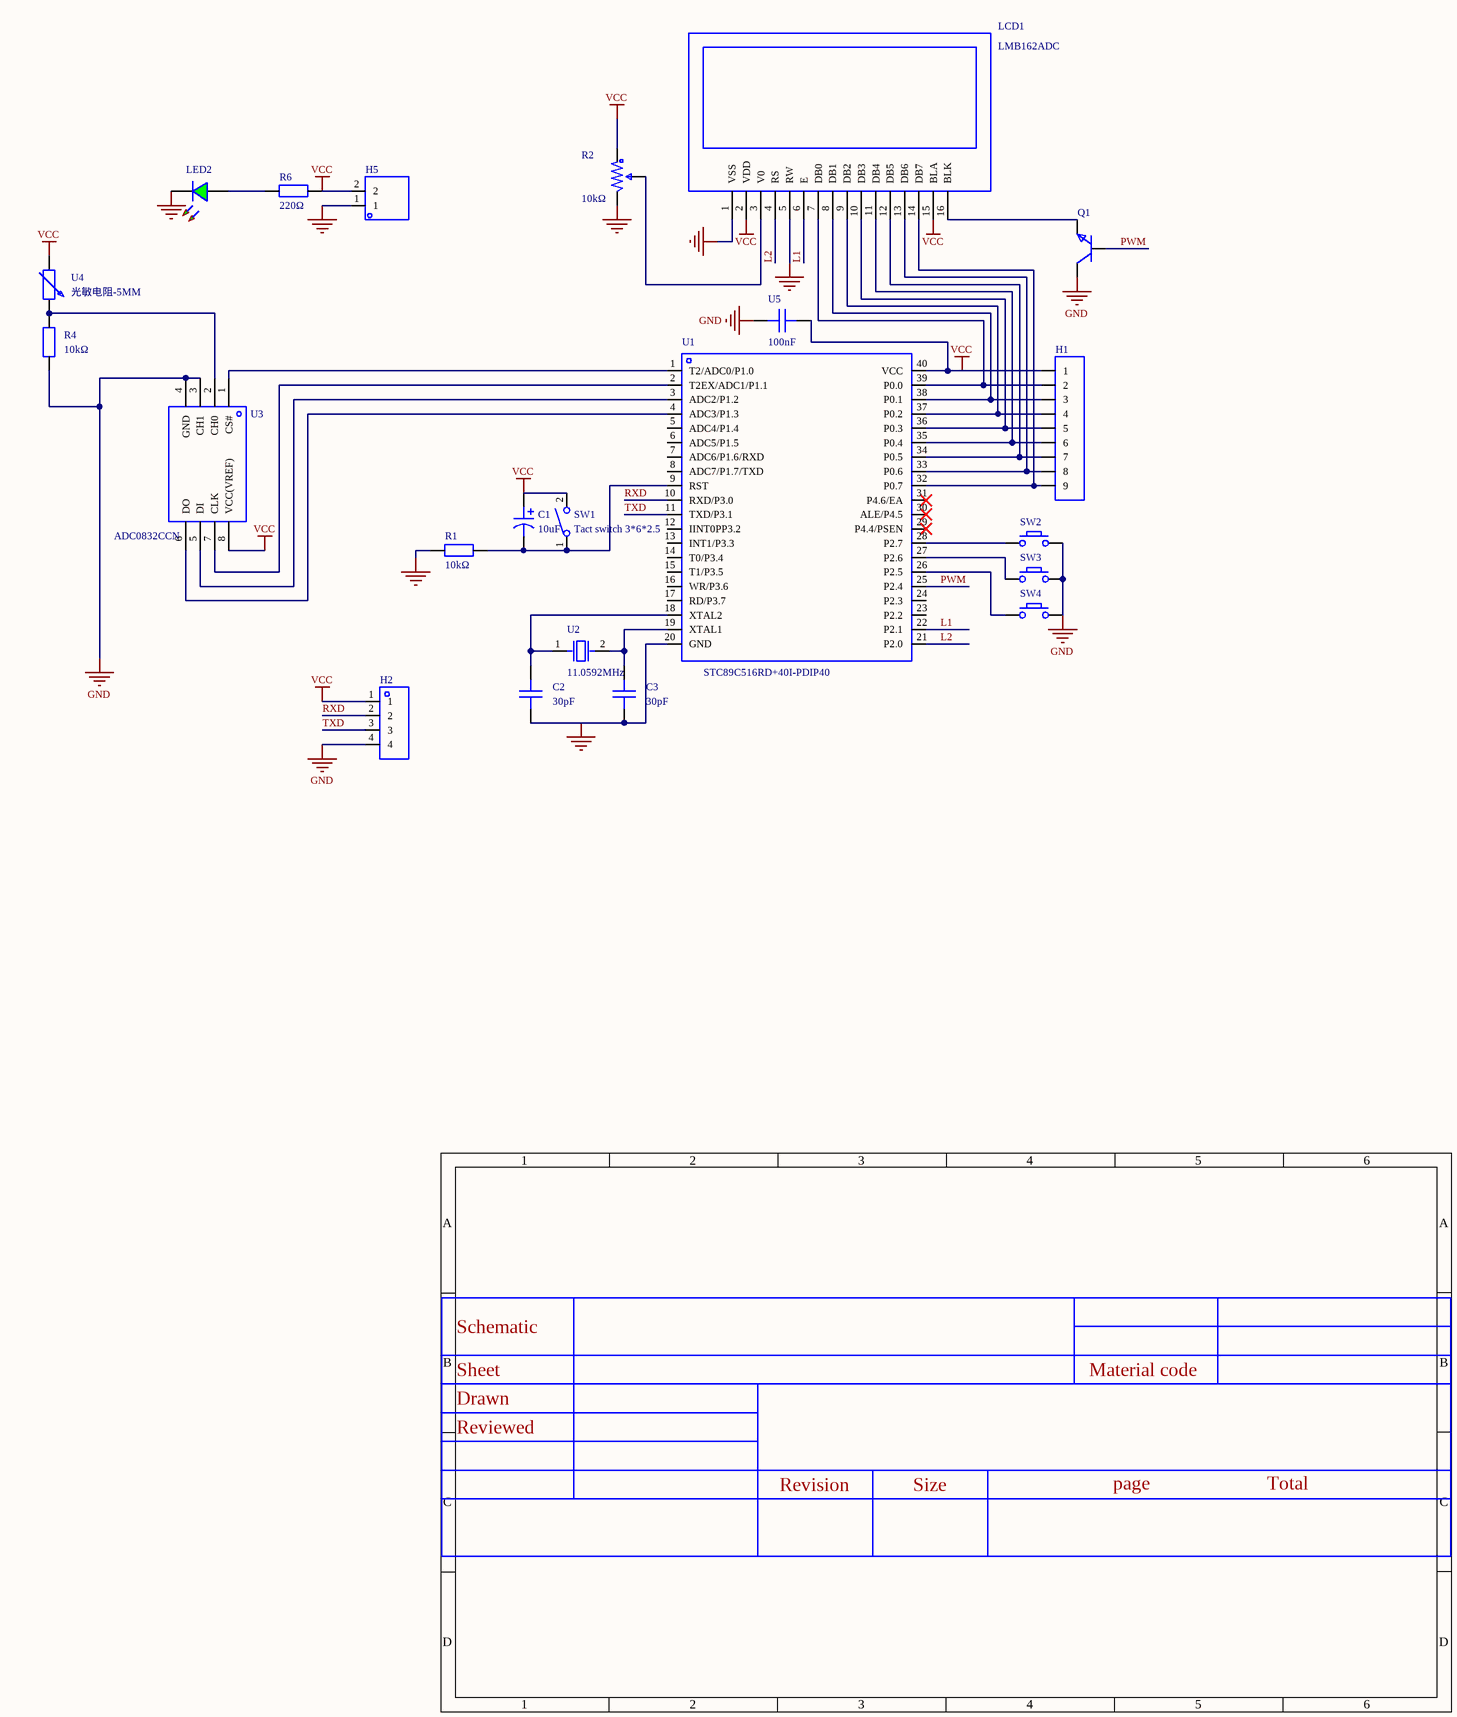
[diagram p0: MISC51926-3.schdoc]
# Altium project MISC51926-2.PrjPcb
1 sheet, 22 parts. Net scope: global (net labels, ports and power ports of the same name join across sheets).
Board file: MISC51926.pcbdoc

## Sheet MISC51926-3.schdoc
size 178 x 98 mm; Version: V1.0; @Project Name: MISC51926; @Page Count: 1; @Update Date: 2026-04-15; @Create Date: 2026-04-15; @Schematic Name: MISC51926; @Page No: 1; @Board Name: MISC51926; @Create Time: 22:37:32; @Update Time: 22:37:32

### Parts
C1  10uF  [CAP-TH_BD5.0-P2.00-D0.8-FD-10UF50VC110GL]
C2  30pF  [CAP-TH_L3.8-W2.5-P2.54-D0.50]
C3  30pF  [CAP-TH_L3.8-W2.5-P2.54-D0.50]
H1  (no value)  [HDR-TH_9P-P2.54-V-F-1]
H2  (no value)  [HDR-TH_4P-P2.54-V-M]
H5  (no value)  [HDR-TH_2P-P2.54-V-M-1]
LCD1  LMB162ADC  [LCD1602]
LED2  (no value)  [LED_TH-3mm]
Q1  (no value)  [S8050_SOT-23]
R1  10kΩ  [Res_1/8W]
R2  10kΩ  [RES-ADJ-SMD_RM065-V1]
R4  10kΩ  [Res_1/8W]
R6  220Ω  [Res_1/8W]
SW1  Tact switch 3*6*2.5  [SW-SMD_L6.0-W3.6-LS8.0]
SW2  (no value)  [Key_TH_3.5x6x4.3]
SW3  (no value)  [Key_TH_3.5x6x4.3]
SW4  (no value)  [Key_TH_3.5x6x4.3]
U1  STC89C516RD+40I-PDIP40  [DIP-40_L52.3-W13.9-P2.54-LS15.2-BL]
U2  11.0592MHz  [HC-49US_L11.0-W4.6-P4.88]
U3  ADC0832CCN  [DIP-8_L9.7-W6.4-P2.54-LS7.6-BL]
U4  光敏电阻-5MM  [RES-TH_L4.9-W4.3-P3.4]
U5  100nF  [CAP-TH_L5.0-W2.5-P5.00-D1.0]

### Nets
GND: C2.1 C3.1 H2.4 H5.1 LCD1.1(VSS) LCD1.5(RW) LED2.2(A) Q1.3 R1.1 R2.3 R4.1 SW2.B SW3.B SW4.B U1.20(GND) U3.3(CH1) U3.4(GND) U5.2
VCC: C1.1 H1.1 H2.1 H5.2 LCD1.2(VDD) LCD1.15(BLA) R2.1 R6.2 SW1.2 U1.40(VCC) U3.8(VCC(VREF)) U4.1 U5.1
L1: LCD1.6(E) U1.22(P2.1)
L2: LCD1.4(RS) U1.21(P2.0)
PWM: Q1.1 U1.25(P2.4)
RXD: H2.2 U1.10(RXD/P3.0)
TXD: H2.3 U1.11(TXD/P3.1)
NetC1_2: C1.2 R1.2 SW1.1 U1.9(RST)
NetC2_2: C2.2 U1.18(XTAL2) U2.1(OSC1)
NetC3_2: C3.2 U1.19(XTAL1) U2.2(OSC2)
NetH1_2: H1.2 LCD1.7(DB0) U1.39(P0.0)
NetH1_3: H1.3 LCD1.8(DB1) U1.38(P0.1)
NetH1_4: H1.4 LCD1.9(DB2) U1.37(P0.2)
NetH1_5: H1.5 LCD1.10(DB3) U1.36(P0.3)
NetH1_6: H1.6 LCD1.11(DB4) U1.35(P0.4)
NetH1_7: H1.7 LCD1.12(DB5) U1.34(P0.5)
NetH1_8: H1.8 LCD1.13(DB6) U1.33(P0.6)
NetH1_9: H1.9 LCD1.14(DB7) U1.32(P0.7)
NetLCD1_3: LCD1.3(V0) R2.2
NetLCD1_16: LCD1.16(BLK) Q1.2
NetLED2_1: LED2.1(C) R6.1
NetR4_2: R4.2 U3.2(CH0) U4.2
NetSW2_A: SW2.A U1.28(P2.7)
NetSW3_A: SW3.A U1.27(P2.6)
NetSW4_A: SW4.A U1.26(P2.5)
NetU1_1: U1.1(T2/ADC0/P1.0) U3.1(CS#)
NetU1_2: U1.2(T2EX/ADC1/P1.1) U3.7(CLK)
NetU1_3: U1.3(ADC2/P1.2) U3.5(DI)
NetU1_4: U1.4(ADC3/P1.3) U3.6(DO)

Not connected (* = marked no-connect by the designer): U1 5(ADC4/P1.4) 6(ADC5/P1.5) 7(ADC6/P1.6/RXD) 8(ADC7/P1.7/TXD) 12(IINT0PP3.2) 13(INT1/P3.3) 14(T0/P3.4) 15(T1/P3.5) 16(WR/P3.6) 17(RD/P3.7) 23(P2.2) 24(P2.3) 29(P4.4/PSEN)* 30(ALE/P4.5)* 31(P4.6/EA)*

### Notes on the sheet
- 2026-04-15
- Schematic
- Sheet
- Material code
- P1
- Reviewed
- Drawn
- 51 project
- Revision
- Size
- page
- Total
- A4
- 1

### Library data of the parts
C1 = 10UF50VC110GL: Capacitance: 10uF; tolerance: ±20%; rated voltage: 50V; ripple current: 120mA@100KHz; equivalent series resistance (ESR): 1.6Ω;; Manufacturer: Econd(米朗电子); AddInBom: yes; Pin Spacing: 2mm; Lifetime: 5000hrs@105℃; Symbol: 10UF50VC110GL; Device: 10UF50VC110GL; LCSC Part Name: 10uF ±20% 50V; SupplierPart: C46867109; ManufacturerPart: 10UF50VC110GL; Supplier Footprint: 插件,D5xL11mm; JLCPCB Part Class: Extended Part; Datasheet: https://item.szlcsc.com/datasheet/10UF50VC110GL/49031974.html; Supplier: LCSC; ConvertToPcb: yes; FootprintName: CAP-TH_BD5.0-P2.00-D0.8-FD-10UF50VC110GL; Value: 10uF; Tolerance: ±20%; Voltage Rating: 50V; Ripple Current: 120mA@100KHz; Equivalent Series Resistance(ESR): 1.6Ω; Diameter: 5mm; Height - Seated (Max): 11mm; Operating Temperature: -40℃~+105℃
C2 C3 = C315C300K3G5TA7301: Capacitance: 30pF; tolerance: ±10%; rated voltage: 25V; temperature coefficient: C0G;; Manufacturer: KEMET(基美); AddInBom: yes; ModelId: 0be8c650c9044d099e9add656cc6dda60819f05c4eef4c71ace90d822a990e87; ModelTransform: 149.606,98.8187,0,0,0,0,0,0,-196.85; Pin Spacing: 2.54mm; Symbol: C315C300K3G5TA7301; Device: C315C300K3G5TA7301; LCSC Part Name: 30pF ±10% 25V; SupplierPart: C2245291; ManufacturerPart: C315C300K3G5TA7301; Supplier Footprint: 插件,P=2.54mm; JLCPCB Part Class: Extended Part; Datasheet: https://item.szlcsc.com/datasheet/C315C300K3G5TA7301/2337370.html; Supplier: LCSC; ConvertToPcb: yes; FootprintName: CAP-TH_L3.8-W2.5-P2.54-D0.50; ModelName: CAP-TH_L3.8-W2.5-P2.54-D0.50; Value: 30pF; Tolerance: ±10%; Voltage Rating: 25V; Temperature Coefficient: C0G
H1 = HDR-F_2.54_1x9P: Symbol: Header-Female-2.54_1x9; AddInBom: yes; ModelId: 3a7016416d904017ac5ead6cc0f14e9c; ModelName: HDR-TH_9P-P2.54-F-LI-1X9P; ModelTransform: 915.746,94.488,0,0,0,0,0,0,-125.984; Device: HDR-F_2.54_1x9P; ConvertToPcb: yes; FootprintName: HDR-TH_9P-P2.54-V-F-1; SupplierPart: C39576; Supplier Footprint: 插件; JLCPCB Part Class: Extended Part
H2 = HDR-M_2.54_1x4P: Symbol: PZ254V-11-04P; 3D Model: 112f4d05e8d64e99ab9a333894bea4f9; 3D Model Transform: 399.999,104.7242,0,0,0,0,0,0,-118.11; ConvertToPcb: yes; ModelName: HDR-TH_4P-P2.54-M-LI-1X4P; Device: HDR-M_2.54_1x4P; Supplier Part: C492403; Supplier Footprint: 插件; AddInBom: yes; FootprintName: HDR-TH_4P-P2.54-V-M
H5 = HDR-M_2.54_1x2P: Symbol: 210S-1*2P L=11.6MMGold-plated black; ConvertToPcb: yes; ModelId: 79b2e9f2d70a4d68a1b7098f27c6d4c5; ModelName: HDR-M-2.54_1x2; ModelTransform: 200,100,0,0,0,0,0,0,-118.11; Device: HDR-M_2.54_1x2P; AddInBom: yes; SupplierPart: C124375; Supplier Footprint: 插件; FootprintName: HDR-TH_2P-P2.54-V-M-1
LCD1 = LMB162ADC: 16x2 character LCD module; AddInBom: yes; ModelId: f9d832f46a914cadb50fc4d4cefd2517; ModelTransform: 3149.6,1417.32,0,0,0,0,0,0,-118.11; Symbol: LMB162ADC; Device: LMB162ADC; LCSC Part Name: LMB162ADC; SupplierPart: C9741; ManufacturerPart: LMB162ADC; Supplier Footprint: SIP; JLCPCB Part Class: Extended Part; Supplier: LCSC; ConvertToPcb: yes; FootprintName: LCD1602; ModelName: LCD1602
LED2 = LED_TH-G_3mm: AddInBom: yes; ModelId: 07c881668c9448ef9b36eb6a2126ca130819f05c4eef4c71ace90d822a990e87; ModelName: LED-TH-3mm_G; ModelTransform: 141.27444,153.32669525336098,354.32999763315956,0,0,0,-5.90551,0,-137.79528; Symbol: LED_TH-G; Device: LED_TH-G_3mm; ConvertToPcb: yes; FootprintName: LED_TH-3mm; Supplier Footprint: 插件
Q1 = S8050_SOT_NPN: Symbol: NPN; ConvertToPcb: yes; ModelId: c62791f0466c4ae2a892c056b845b0ca0819f05c4eef4c71ace90d822a990e87; ModelName: SOT-23-3P_L2.9-W1.3-H1.0-LS2.4-P0.95; ModelTransform: 98.6,114.12,41.29,180,0,0,0,0,-3; Device: S8050_SOT_NPN; AddInBom: yes; Supplier Footprint: SOT-23; FootprintName: S8050_SOT-23
R1 R4 R6 = Res_AXIAL-1/8W: Symbol: Resistor; ConvertToPcb: yes; ModelId: b2b5ae7ae4c642178fe0039925c86a3f0819f05c4eef4c71ace90d822a990e87; ModelName: RES-TH_BD1.8-L3.2-P7.20-D0.4; ModelTransform: 282.86,66.88,253.09,0,0,0,0,0,-191; Device: Res_AXIAL-1/8W; AddInBom: yes; Supplier Footprint: 轴向引线; FootprintName: Res_1/8W
  R1 R4: Value: 10kΩ
  R6: Value: 220Ω
R2 = RM065-103(10K): Resistance: 10kΩ; tolerance: ±25%; power: 100mW;; Manufacturer: BOCHEN(博晨); AddInBom: yes; ModelId: c816c2b7942147f5a832150e8ef6960c0819f05c4eef4c71ace90d822a990e87; ModelTransform: 255.905,283.464,0,0,0,0,0.025,-3.937,-157.48; Voltage Rating: 50V; Symbol: RM065-103(10K); Device: RM065-103(10K); LCSC Part Name: 10kΩ ±25%; SupplierPart: C5205021; ManufacturerPart: RM065-103(10K); Supplier Footprint: 插件,7.3x6.4mm; JLCPCB Part Class: Extended Part; Datasheet: https://item.szlcsc.com/datasheet/RM065-103(10K)/5896379.html; Supplier: LCSC; ConvertToPcb: yes; FootprintName: RES-ADJ-SMD_RM065-V1; ModelName: RES-ADJ-SMD_RM065-V1; Value: 10kΩ; Tolerance: ±25%; Power(Watts): 100mW
SW1 = 轻触按键3*6*2.5: AddInBom: yes; ModelId: 5cda64a5897044e48badc24f5aa7d420; ModelName: SW-SMD_L6.0-W3.6-H2.5-LS8.0; ModelTransform: 314.96,141.732,0,0,0,0,0,0,0; Symbol: Tact switch 3*6*2.5; Device: Tact switch 3*6*2.5; LCSC Part Name: 轻触按键3*6*2.5; SupplierPart: C9900013040; ManufacturerPart: 轻触按键3*6*2.5; Supplier Footprint: KEY; JLCPCB Part Class: Extended Part; Supplier: LCSC; ConvertToPcb: yes; FootprintName: SW-SMD_L6.0-W3.6-LS8.0
SW2-SW4 = Key_TH_3.5x6x4.3: ConvertToPcb: yes; ModelId: c3523f9014d949d7ba5445190a3178990819f05c4eef4c71ace90d822a990e87; ModelName: SW-TH_L6.0-W3.5-H5.0-P6.5; ModelTransform: 308.49,137.8,335.08,0,0,0,0,0,-129.92; Symbol: Key_TH_3.5x6x4.3; Device: Key_TH_3.5x6x4.3; AddInBom: yes; Supplier Footprint: 插件; FootprintName: Key_TH_3.5x6x4.3
U1 = STC89C516RD+40I-PDIP40: CPU core: 51 series; program storage capacity: 61KB; RAM total capacity: 1.25KB; GPIO port count: 35; operating voltage range: 3.5V~5.5V; CPU max frequency: -; program memory type: FLASH;; Manufacturer: STC(宏晶); AddInBom: yes; ModelId: 16d4686a009b4ddca948f91eddb57b14; ModelName: DIP-40_L52.3-W13.8-H4.0-LS15.24-P2.54; ModelTransform: 2059.051,615.743,0,0,0,0,0,0,-129.921; GPIO Ports Number: 35; 16Bit Timer: 3; UART/USART: 1; Peripheral/Function: Watchdog; Symbol: STC89C516RD+40I-PDIP40; Device: STC89C516RD+40I-PDIP40; LCSC Part Name: STC89C516RD+40I-PDIP40; SupplierPart: C52225; ManufacturerPart: STC89C516RD+40I-PDIP40; Supplier Footprint: DIP-40; JLCPCB Part Class: Extended Part; Datasheet: https://atta.szlcsc.com/upload/public/pdf/source/20180614/C87831_BBAF7FB8B286C29ACE4E9B180C033FEC.pdf; Supplier: LCSC; ConvertToPcb: yes; FootprintName: DIP-40_L52.3-W13.9-P2.54-LS15.2-BL; CPU Core: 51 series; Program Storage Size: 61KB; RAM Size: 1.25KB; Operating Voltage Range: 3.5V~5.5V; CPU Maximum Speed: -; Program Memory Type: FLASH; Operating Temperature Range: -40℃~+85℃; ADC (Bit): -; DAC (Bit): -; PWM (Bit): -; 8Bit Timer: -; 32Bit Timer: -; CAN: -; I2C: -; I2S: -; SPI: -; Universal Serial Bus: -; Internal Comparator: -; communication protocol: -; Watchdog: Yes; Real-Time Clock: -; Infrared Data Association: -; Low-Voltage Detect: -; CCP Capture/Compare: -; Secure Digital Input and Output: -; Direct Memory Access: -; Internal Oscillator: -
U2 = ECS-120-S-4: Frequency: 12MHz; normal temperature frequency tolerance: ±30ppm; external load capacitance: -; frequency stability (full temperature): ±50ppm;; Manufacturer: ECS; AddInBom: yes; ModelId: 59d05c800eee432cb051aa4925461fda; ModelName: HC-49US_L11.0-W4.7-H3.5-P4.88; ModelTransform: 432.44473,183.0705,0,0,0,0,0,0,-137.795; Equivalent Series Resistance (ESR): 60Ω; Symbol: ECS-120-S-4; Value: 11.0592MHz; Device: ECS-120-S-4; LCSC Part Name: 12MHz ±30ppm; ManufacturerPart: ECS-120-S-4; Supplier Footprint: HC-49S; JLCPCB Part Class: Extended Part; Datasheet: https://atta.szlcsc.com/upload/public/pdf/source/20210402/81F084B668D60DFAE850A61100CCABAF.pdf; Supplier: LCSC; ConvertToPcb: yes; FootprintName: HC-49US_L11.0-W4.6-P4.88; Normal temperature Frequency Tolerance: ±30ppm; External load capacitor: -; Frequency Stability(Full temperature range): ±50ppm; Operating Temperature: -10℃~+70℃
U3 = ADC0832CCN: AddInBom: yes; ModelId: 5746b540d01a4d1b9eb6b4f989297bc70819f05c4eef4c71ace90d822a990e87; ModelName: DIP-8_L9.8-W6.6-H3.5-LS7.62-P2.54; ModelTransform: 385.826,311.8104,0,0,0,0,0,0,-118.11; Symbol: ADC0832CCN; Device: ADC0832CCN; LCSC Part Name: ADC0832CCN; SupplierPart: C10915; ManufacturerPart: ADC0832CCN; Supplier Footprint: DIP-8; JLCPCB Part Class: Extended Part; Supplier: LCSC; ConvertToPcb: yes; FootprintName: DIP-8_L9.7-W6.4-P2.54-LS7.6-BL
U4 = 光敏电阻-5MM: AddInBom: yes; ModelId: 8cda4899688949e78503a56fe341541c0819f05c4eef4c71ace90d822a990e87; ModelTransform: 169.291,200.6107,0,90,0,0,0,0,-196.85; Symbol: 光敏电阻-5MM; Device: 光敏电阻-5MM; LCSC Part Name: 光敏电阻-5MM; SupplierPart: C9900003115; ManufacturerPart: 光敏电阻-5MM; Supplier Footprint: RES-TH_4.3X4.9X3.37P; JLCPCB Part Class: Extended Part; Supplier: LCSC; ConvertToPcb: yes; FootprintName: RES-TH_L4.9-W4.3-P3.4; ModelName: RES-TH_L4.9-W4.3-P3.4
U5 = 100nF: Symbol: 100NF_C9900015256; AddInBom: yes; ModelId: 08e3d7481fc7486bb1b263873f51e1e10819f05c4eef4c71ace90d822a990e87; ModelName: CAP-TH_BD5.0-W2.5-P5.08; ModelTransform: 224.652,98.425,0,0,0,0,-0.005,0,-137.795; Device: 100nF; LCSC Part Name: 100nF; SupplierPart: C9900015256; ManufacturerPart: 100nF; Supplier Footprint: CAP-TH_L5.0-W2.5-P5.00-D1.0; JLCPCB Part Class: Extended Part; Supplier: LCSC; ConvertToPcb: yes; FootprintName: CAP-TH_L5.0-W2.5-P5.00-D1.0